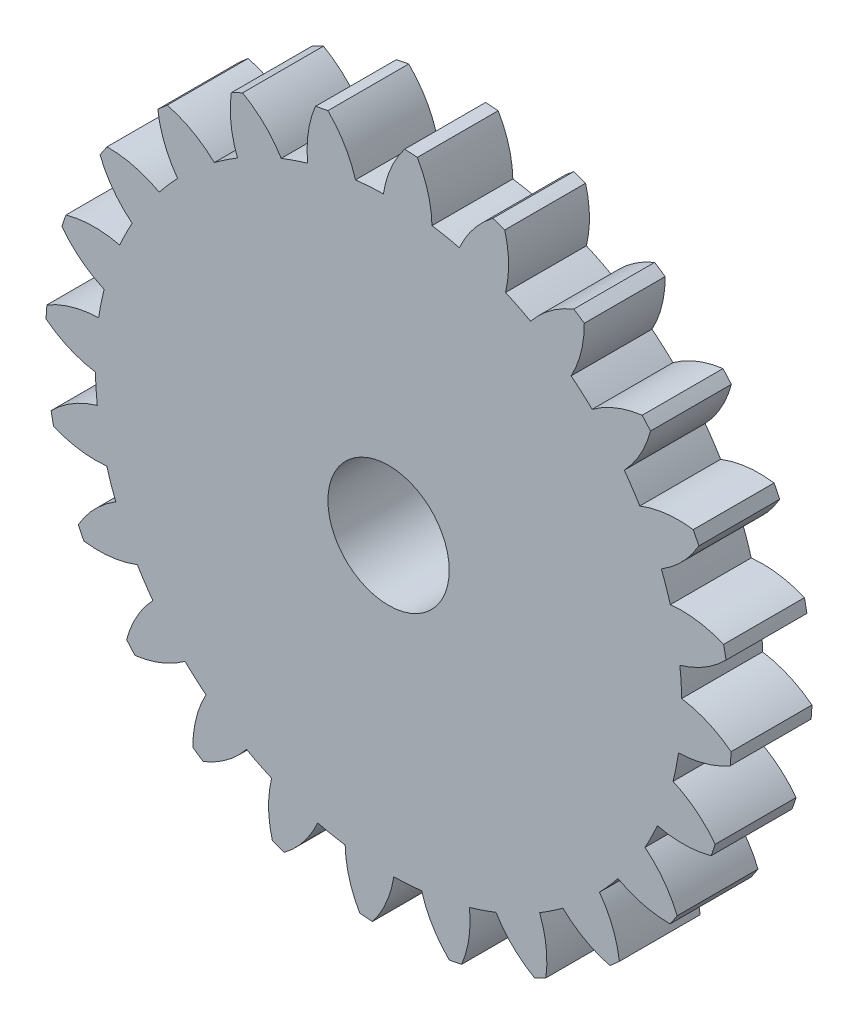
from build123d import *

# Parameters (mm, degrees)
SKETCH1_R           = 7.25
BOSS_EXTRUDE1_DEPTH = 2
SKETCH3_R           = 4.70622852
SKETCH4_R           = 2.420674735
SKETCH5_R           = 2.420674735
BOSS_EXTRUDE3_DEPTH = 1
FILLET1_R           = 0.3
BOSS_EXTRUDE4_DEPTH = 2
CIRPATTERN2_COUNT   = 24
SKETCH6_R           = 1.5
CUT_EXTRUDE1_DEPTH  = 10


with BuildPart() as part:
    # Sketch1 → Boss-Extrude1 (new body)
    with BuildSketch(Plane.XY):
        Circle(SKETCH1_R)
    extrude(amount=BOSS_EXTRUDE1_DEPTH)

    # Sketch3 → Loft1 section 0
    with BuildSketch(Plane(origin=(0, 0, 0), x_dir=(-1, 0, 0), z_dir=(0, 0, -1))):
        Circle(SKETCH3_R)
    # Sketch4 → Loft1 section 1
    with BuildSketch(Plane(origin=(0, 0, -0.8), x_dir=(-1, 0, 0), z_dir=(0, 0, -1))):
        Circle(SKETCH4_R)
    loft()

    # Sketch5 → Boss-Extrude3 (add)
    with BuildSketch(Plane(origin=(0, 0, -0.8), x_dir=(-1, 0, 0), z_dir=(0, 0, -1))):
        Circle(SKETCH5_R)
    extrude(amount=BOSS_EXTRUDE3_DEPTH)

    # Fillet1
    fillet1_edges = [part.edges().sort_by_distance(p)[0] for p in [
        (2.420674735, 0, -1.8),
        (2.420674735, 0, -0.8),
    ]]
    fillet(fillet1_edges, radius=FILLET1_R)

    # Sketch2 → Boss-Extrude4 (add)
    with BuildSketch(Plane.XY.offset(2)):
        with BuildLine():
            ThreePointArc((0.710649734, 8.450170232), (0.554618536, 8.461843669), (0.398398517, 8.470636258))
            ThreePointArc((0.398398517, 8.470636258), (-0.000769738, 7.747882363), (-0.158188639, 6.937371549))
            ThreePointArc((-0.158188639, 6.937371549), (0.45384375, 6.924317548), (1.062344006, 6.857373613))
            ThreePointArc((1.062344006, 6.857373613), (1.012064735, 7.681497684), (0.710649734, 8.450170232))
        make_face()
    boss_extrude4 = extrude(amount=-BOSS_EXTRUDE4_DEPTH)

    # CirPattern2: Boss-Extrude4 ×24 about axis
    cirpattern2_axis = Axis((0, 0, 0), (0, 0, 1))
    for i in range(1, CIRPATTERN2_COUNT):
        add(boss_extrude4.rotate(cirpattern2_axis, i * 360 / CIRPATTERN2_COUNT))

    # Sketch6 → Cut-Extrude1 (cut)
    with BuildSketch(Plane(origin=(0, 0, -1.8), x_dir=(-1, 0, 0), z_dir=(0, 0, -1))):
        Circle(SKETCH6_R)
    extrude(amount=-CUT_EXTRUDE1_DEPTH, mode=Mode.SUBTRACT)


solid = part.part
